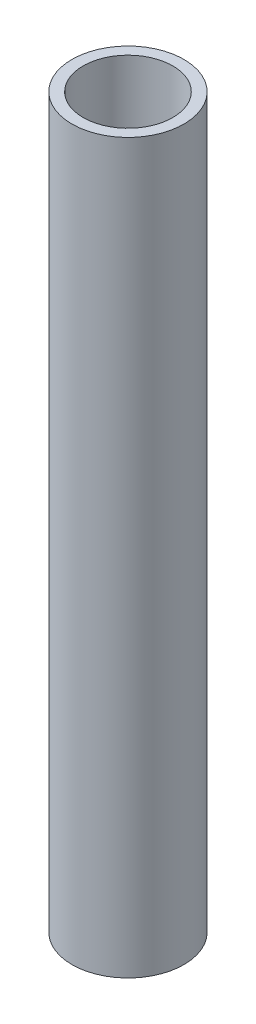
SolidWorks part; units mm, degrees
material "20 steel"
ref_plane "Front Plane" through (0, 0, 0) normal (0, 0, 1) x (1, 0, 0)
ref_plane "Top Plane" through (0, 0, 0) normal (0, 1, 0) x (1, 0, 0)
ref_plane "Right Plane" through (0, 0, 0) normal (1, 0, 0) x (0, 0, -1)
other "Configuration Table"
sketch "Sketch1" plane through (0, 0, 0) normal (0, 1, 0) x (1, 0, 0)
  circle A0 centre (0, 0) radius 8
  circle A1 centre (0, 0) radius 10
  dimension "D1" = 20
  dimension "D2" = 16
extrude "Boss-Extrude1" add sketch "Sketch1" along normal blind 130
